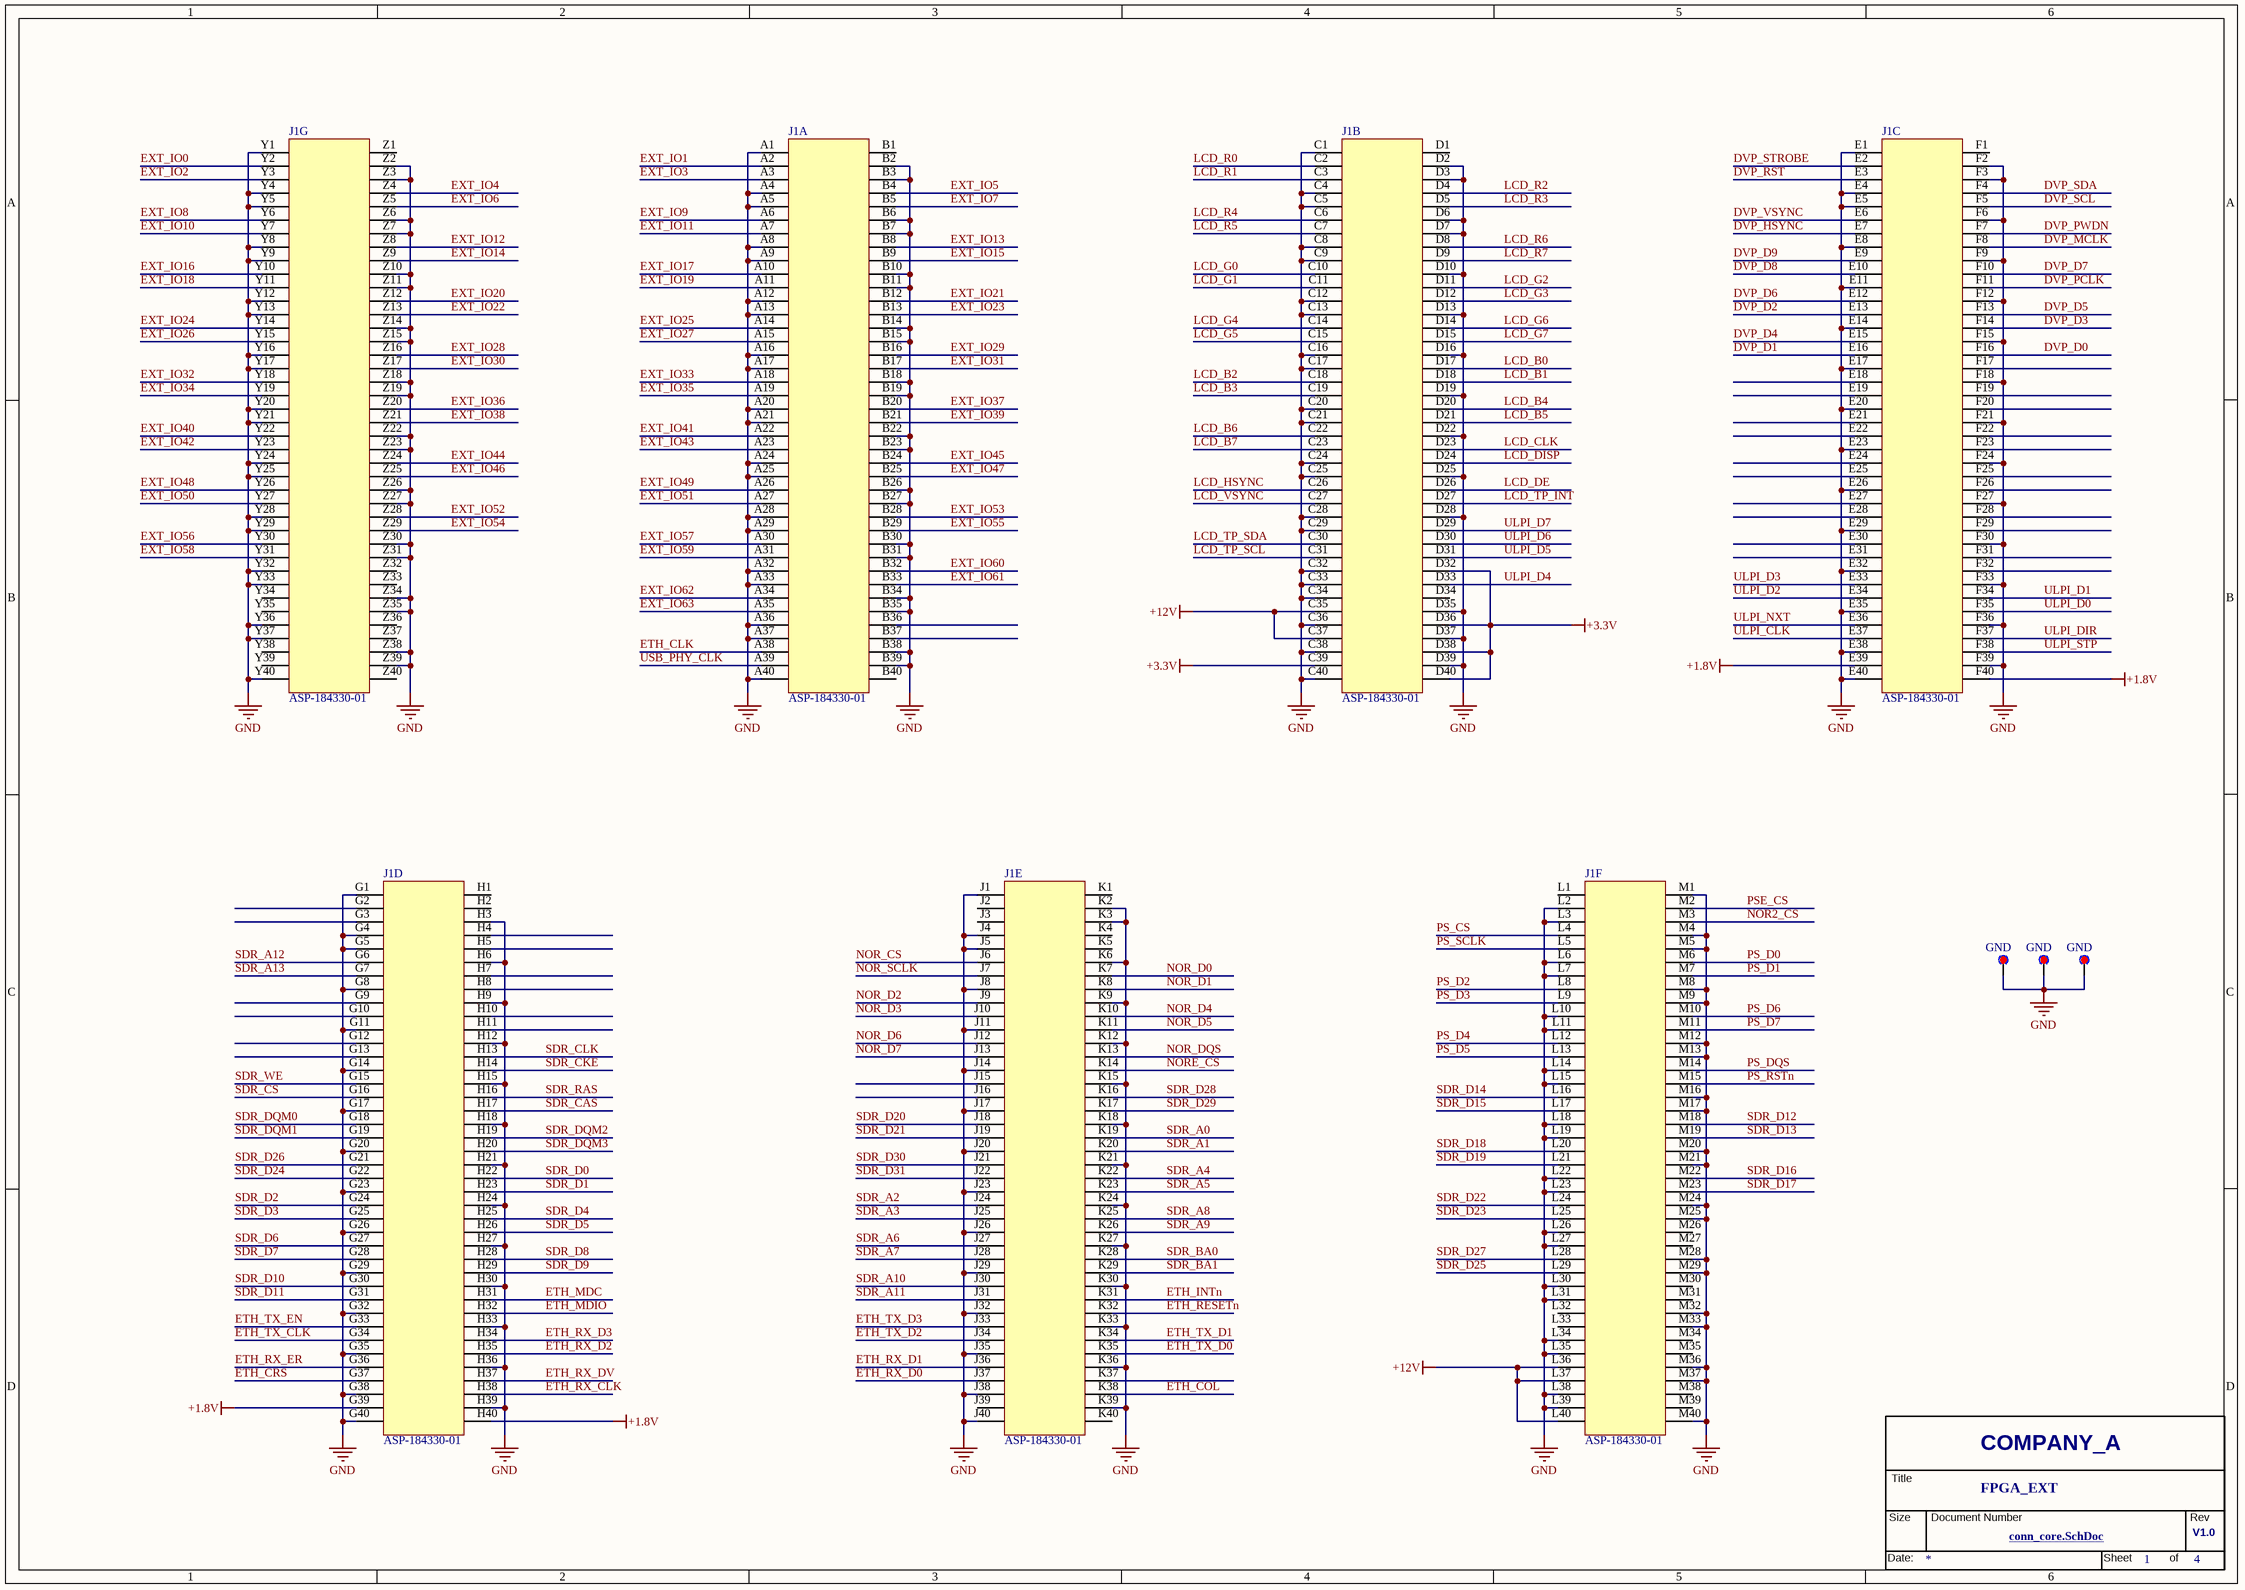
[diagram p0: MISC105414-3.SchDoc]
# Altium project MISC105414-4.PrjPcb (part 1 of 3)
4 sheets, 256 parts. Net scope: global (net labels, ports and power ports of the same name join across sheets).
Board file: MISC105414.PcbDoc
Sheets:
  MISC105414-3.SchDoc
  MISC105414-2.SchDoc
  MISC105414-7.SchDoc
  MISC105414-8.SchDoc

## Sheet MISC105414-3.SchDoc
size 420 x 297 mm; DocumentNumber: MISC105414; SheetNumber: 1; SheetTotal: 4

### Parts
(Parts that share a designator on the sheet are numbered #1, #2 ... from top to bottom, then left to right.)
*?#1  Page Count: 4  Page Number: 1  OrgName: COMPANY_A  Title: FPGA_EXT  RevCode: V1.0  Doc: conn_core.SchDoc  (hidden comment: TitleBlock_YHSCH)  (graphical)
J1  ASP-184330-01  [ASP-184330-01_Bottom]  (parts A,B,C,D,E,F,G of 7)
TP1  GND  [FZ_TP-Via]
TP2  GND  [FZ_TP-Via]
TP3  GND  [FZ_TP-Via]

### Nets
+1.8V: J1.E39(P) J1.F40(P) J1.G39(P) J1.H40(P)
+3.3V: J1.C39(P) J1.D32(P) J1.D36(P) J1.D38(P) J1.D40(P)
+12V: J1.C35(P) J1.C37(P) J1.L36(P) J1.L37(P) J1.L40(P)
GND: J1.A1(P) J1.A4(P) J1.A5(P) J1.A8(P) J1.A9(P) J1.A12(P) J1.A13(P) J1.A16(P) J1.A17(P) J1.A20(P) J1.A21(P) J1.A24(P) J1.A25(P) J1.A28(P) J1.A29(P) J1.A32(P) J1.A33(P) J1.A36(P) J1.A37(P) J1.A40(P) J1.B2(P) J1.B3(P) J1.B6(P) J1.B7(P) J1.B10(P) J1.B11(P) J1.B14(P) J1.B15(P) J1.B18(P) J1.B19(P) J1.B22(P) J1.B23(P) J1.B26(P) J1.B27(P) J1.B30(P) J1.B31(P) J1.B34(P) J1.B35(P) J1.B38(P) J1.B39(P) J1.C1(P) J1.C4(P) J1.C5(P) J1.C8(P) J1.C9(P) J1.C12(P) J1.C13(P) J1.C16(P) J1.C17(P) J1.C20(P) J1.C21(P) J1.C24(P) J1.C25(P) J1.C28(P) J1.C29(P) J1.C32(P) J1.C33(P) J1.C34(P) J1.C36(P) J1.C38(P) J1.C40(P) J1.D2(P) J1.D3(P) J1.D6(P) J1.D7(P) J1.D10(P) J1.D13(P) J1.D16(P) J1.D19(P) J1.D22(P) J1.D25(P) J1.D28(P) J1.D35(P) J1.D37(P) J1.D39(P) J1.E1(P) J1.E4(P) J1.E5(P) J1.E8(P) J1.E11(P) J1.E14(P) J1.E17(P) J1.E20(P) J1.E23(P) J1.E26(P) J1.E29(P) J1.E32(P) J1.E35(P) J1.E38(P) J1.E40(P) J1.F2(P) J1.F3(P) J1.F6(P) J1.F9(P) J1.F12(P) J1.F15(P) J1.F18(P) J1.F21(P) J1.F24(P) J1.F27(P) J1.F30(P) J1.F33(P) J1.F36(P) J1.F39(P) J1.G1(P) J1.G4(P) J1.G5(P) J1.G8(P) J1.G11(P) J1.G14(P) J1.G17(P) J1.G20(P) J1.G23(P) J1.G26(P) J1.G29(P) J1.G32(P) J1.G35(P) J1.G38(P) J1.G40(P) J1.H3(P) J1.H6(P) J1.H9(P) J1.H12(P) J1.H15(P) J1.H18(P) J1.H21(P) J1.H24(P) J1.H27(P) J1.H30(P) J1.H33(P) J1.H36(P) J1.H39(P) J1.J1(P) J1.J4(P) J1.J5(P) J1.J8(P) J1.J11(P) J1.J14(P) J1.J17(P) J1.J20(P) J1.J23(P) J1.J26(P) J1.J29(P) J1.J32(P) J1.J35(P) J1.J38(P) J1.J40(P) J1.K2(P) J1.K3(P) J1.K6(P) J1.K9(P) J1.K12(P) J1.K15(P) J1.K18(P) J1.K21(P) J1.K24(P) J1.K27(P) J1.K30(P) J1.K33(P) J1.K36(P) J1.K39(P) J1.L2(P) J1.L3(P) J1.L6(P) J1.L7(P) J1.L10(P) J1.L11(P) J1.L14(P) J1.L15(P) J1.L18(P) J1.L19(P) J1.L22(P) J1.L23(P) J1.L26(P) J1.L27(P) J1.L30(P) J1.L31(P) J1.L34(P) J1.L35(P) J1.L38(P) J1.L39(P) J1.M1(P) J1.M4(P) J1.M5(P) J1.M8(P) J1.M9(P) J1.M12(P) J1.M13(P) J1.M16(P) J1.M17(P) J1.M20(P) J1.M21(P) J1.M24(P) J1.M25(P) J1.M28(P) J1.M29(P) J1.M32(P) J1.M33(P) J1.M36(P) J1.M37(P) J1.M40(P) J1.Y1(P) J1.Y4(P) J1.Y5(P) J1.Y8(P) J1.Y9(P) J1.Y12(P) J1.Y13(P) J1.Y16(P) J1.Y17(P) J1.Y20(P) J1.Y21(P) J1.Y24(P) J1.Y25(P) J1.Y28(P) J1.Y29(P) J1.Y32(P) J1.Y33(P) J1.Y36(P) J1.Y37(P) J1.Y40(P) J1.Z2(P) J1.Z3(P) J1.Z6(P) J1.Z7(P) J1.Z10(P) J1.Z11(P) J1.Z14(P) J1.Z15(P) J1.Z18(P) J1.Z19(P) J1.Z22(P) J1.Z23(P) J1.Z26(P) J1.Z27(P) J1.Z30(P) J1.Z31(P) J1.Z34(P) J1.Z35(P) J1.Z38(P) J1.Z39(P) TP1.1 TP2.1 TP3.1
DVP_D0: J1.F16(P)
DVP_D1: J1.E16(P)
DVP_D2: J1.E13(P)
DVP_D3: J1.F14(P)
DVP_D4: J1.E15(P)
DVP_D5: J1.F13(P)
DVP_D6: J1.E12(P)
DVP_D7: J1.F10(P)
DVP_D8: J1.E10(P)
DVP_D9: J1.E9(P)
DVP_HSYNC: J1.E7(P)
DVP_MCLK: J1.F8(P)
DVP_PCLK: J1.F11(P)
DVP_PWDN: J1.F7(P)
DVP_RST: J1.E3(P)
DVP_SCL: J1.F5(P)
DVP_SDA: J1.F4(P)
DVP_STROBE: J1.E2(P)
DVP_VSYNC: J1.E6(P)
ETH_CLK: J1.A38(P)
ETH_COL: J1.K38(P)
ETH_CRS: J1.G37(P)
ETH_INTn: J1.K31(P)
ETH_MDC: J1.H31(P)
ETH_MDIO: J1.H32(P)
ETH_RESETn: J1.K32(P)
ETH_RX_CLK: J1.H38(P)
ETH_RX_D0: J1.J37(P)
ETH_RX_D1: J1.J36(P)
ETH_RX_D2: J1.H35(P)
ETH_RX_D3: J1.H34(P)
ETH_RX_DV: J1.H37(P)
ETH_RX_ER: J1.G36(P)
ETH_TX_CLK: J1.G34(P)
ETH_TX_D0: J1.K35(P)
ETH_TX_D1: J1.K34(P)
ETH_TX_D2: J1.J34(P)
ETH_TX_D3: J1.J33(P)
ETH_TX_EN: J1.G33(P)
EXT_IO0: J1.Y2(P)
EXT_IO1: J1.A2(P)
EXT_IO2: J1.Y3(P)
EXT_IO3: J1.A3(P)
EXT_IO4: J1.Z4(P)
EXT_IO5: J1.B4(P)
EXT_IO6: J1.Z5(P)
EXT_IO7: J1.B5(P)
EXT_IO8: J1.Y6(P)
EXT_IO9: J1.A6(P)
EXT_IO10: J1.Y7(P)
EXT_IO11: J1.A7(P)
EXT_IO12: J1.Z8(P)
EXT_IO13: J1.B8(P)
EXT_IO14: J1.Z9(P)
EXT_IO15: J1.B9(P)
EXT_IO16: J1.Y10(P)
EXT_IO17: J1.A10(P)
EXT_IO18: J1.Y11(P)
EXT_IO19: J1.A11(P)
EXT_IO20: J1.Z12(P)
EXT_IO21: J1.B12(P)
EXT_IO22: J1.Z13(P)
EXT_IO23: J1.B13(P)
EXT_IO24: J1.Y14(P)
EXT_IO25: J1.A14(P)
EXT_IO26: J1.Y15(P)
EXT_IO27: J1.A15(P)
EXT_IO28: J1.Z16(P)
EXT_IO29: J1.B16(P)
EXT_IO30: J1.Z17(P)
EXT_IO31: J1.B17(P)
EXT_IO32: J1.Y18(P)
EXT_IO33: J1.A18(P)
EXT_IO34: J1.Y19(P)
EXT_IO35: J1.A19(P)
EXT_IO36: J1.Z20(P)
EXT_IO37: J1.B20(P)
EXT_IO38: J1.Z21(P)
EXT_IO39: J1.B21(P)
EXT_IO40: J1.Y22(P)
EXT_IO41: J1.A22(P)
EXT_IO42: J1.Y23(P)
EXT_IO43: J1.A23(P)
EXT_IO44: J1.Z24(P)
EXT_IO45: J1.B24(P)
EXT_IO46: J1.Z25(P)
EXT_IO47: J1.B25(P)
EXT_IO48: J1.Y26(P)
EXT_IO49: J1.A26(P)
EXT_IO50: J1.Y27(P)
EXT_IO51: J1.A27(P)
EXT_IO52: J1.Z28(P)
EXT_IO53: J1.B28(P)
EXT_IO54: J1.Z29(P)
EXT_IO55: J1.B29(P)
EXT_IO56: J1.Y30(P)
EXT_IO57: J1.A30(P)
EXT_IO58: J1.Y31(P)
EXT_IO59: J1.A31(P)
EXT_IO60: J1.B32(P)
EXT_IO61: J1.B33(P)
EXT_IO62: J1.A34(P)
EXT_IO63: J1.A35(P)
LCD_B0: J1.D17(P)
LCD_B1: J1.D18(P)
LCD_B2: J1.C18(P)
LCD_B3: J1.C19(P)
LCD_B4: J1.D20(P)
LCD_B5: J1.D21(P)
LCD_B6: J1.C22(P)
LCD_B7: J1.C23(P)
LCD_CLK: J1.D23(P)
LCD_DE: J1.D26(P)
LCD_DISP: J1.D24(P)
LCD_G0: J1.C10(P)
LCD_G1: J1.C11(P)
LCD_G2: J1.D11(P)
LCD_G3: J1.D12(P)
LCD_G4: J1.C14(P)
LCD_G5: J1.C15(P)
LCD_G6: J1.D14(P)
LCD_G7: J1.D15(P)
LCD_HSYNC: J1.C26(P)
LCD_R0: J1.C2(P)
LCD_R1: J1.C3(P)
LCD_R2: J1.D4(P)
LCD_R3: J1.D5(P)
LCD_R4: J1.C6(P)
LCD_R5: J1.C7(P)
LCD_R6: J1.D8(P)
LCD_R7: J1.D9(P)
LCD_TP_INT: J1.D27(P)
LCD_TP_SCL: J1.C31(P)
LCD_TP_SDA: J1.C30(P)
LCD_VSYNC: J1.C27(P)
NOR2_CS: J1.M3(P)
NOR_CS: J1.J6(P)
NOR_D0: J1.K7(P)
NOR_D1: J1.K8(P)
NOR_D2: J1.J9(P)
NOR_D3: J1.J10(P)
NOR_D4: J1.K10(P)
NOR_D5: J1.K11(P)
NOR_D6: J1.J12(P)
NOR_D7: J1.J13(P)
NOR_DQS: J1.K13(P)
NOR_SCLK: J1.J7(P)
NORE_CS: J1.K14(P)
PS_CS: J1.L4(P)
PS_D0: J1.M6(P)
PS_D1: J1.M7(P)
PS_D2: J1.L8(P)
PS_D3: J1.L9(P)
PS_D4: J1.L12(P)
PS_D5: J1.L13(P)
PS_D6: J1.M10(P)
PS_D7: J1.M11(P)
PS_DQS: J1.M14(P)
PS_RSTn: J1.M15(P)
PS_SCLK: J1.L5(P)
PSE_CS: J1.M2(P)
SDR_A0: J1.K19(P)
SDR_A1: J1.K20(P)
SDR_A2: J1.J24(P)
SDR_A3: J1.J25(P)
SDR_A4: J1.K22(P)
SDR_A5: J1.K23(P)
SDR_A6: J1.J27(P)
SDR_A7: J1.J28(P)
SDR_A8: J1.K25(P)
SDR_A9: J1.K26(P)
SDR_A10: J1.J30(P)
SDR_A11: J1.J31(P)
SDR_A12: J1.G6(P)
SDR_A13: J1.G7(P)
SDR_BA0: J1.K28(P)
SDR_BA1: J1.K29(P)
SDR_CAS: J1.H17(P)
SDR_CKE: J1.H14(P)
SDR_CLK: J1.H13(P)
SDR_CS: J1.G16(P)
SDR_D0: J1.H22(P)
SDR_D1: J1.H23(P)
SDR_D2: J1.G24(P)
SDR_D3: J1.G25(P)
SDR_D4: J1.H25(P)
SDR_D5: J1.H26(P)
SDR_D6: J1.G27(P)
SDR_D7: J1.G28(P)
SDR_D8: J1.H28(P)
SDR_D9: J1.H29(P)
SDR_D10: J1.G30(P)
SDR_D11: J1.G31(P)
SDR_D12: J1.M18(P)
SDR_D13: J1.M19(P)
SDR_D14: J1.L16(P)
SDR_D15: J1.L17(P)
SDR_D16: J1.M22(P)
SDR_D17: J1.M23(P)
SDR_D18: J1.L20(P)
SDR_D19: J1.L21(P)
SDR_D20: J1.J18(P)
SDR_D21: J1.J19(P)
SDR_D22: J1.L24(P)
SDR_D23: J1.L25(P)
SDR_D24: J1.G22(P)
SDR_D25: J1.L29(P)
SDR_D26: J1.G21(P)
SDR_D27: J1.L28(P)
SDR_D28: J1.K16(P)
SDR_D29: J1.K17(P)
SDR_D30: J1.J21(P)
SDR_D31: J1.J22(P)
SDR_DQM0: J1.G18(P)
SDR_DQM1: J1.G19(P)
SDR_DQM2: J1.H19(P)
SDR_DQM3: J1.H20(P)
SDR_RAS: J1.H16(P)
SDR_WE: J1.G15(P)
ULPI_CLK: J1.E37(P)
ULPI_D0: J1.F35(P)
ULPI_D1: J1.F34(P)
ULPI_D2: J1.E34(P)
ULPI_D3: J1.E33(P)
ULPI_D4: J1.D33(P)
ULPI_D5: J1.D31(P)
ULPI_D6: J1.D30(P)
ULPI_D7: J1.D29(P)
ULPI_DIR: J1.F37(P)
ULPI_NXT: J1.E36(P)
ULPI_STP: J1.F38(P)
USB_PHY_CLK: J1.A39(P)

Not connected (* = marked no-connect by the designer): J1 B1(P) B36(P) B37(P) B40(P) D1(P) D34(P) E18(P) E19(P) E21(P) E22(P) E24(P) E25(P) E27(P) E28(P) E30(P) E31(P) F1(P) F17(P) F19(P) F20(P) F22(P) F23(P) F25(P) F26(P) F28(P) F29(P) F31(P) F32(P) G2(P) G3(P) G9(P) G10(P) G12(P) G13(P) H1(P) H2(P) H4(P) H5(P) H7(P) H8(P) H10(P) H11(P) J2(P) J3(P) J15(P) J16(P) J39(P) K1(P) K4(P) K5(P) K37(P) K40(P) L1(P) L32(P) L33(P) M26(P) M27(P) M30(P) M31(P) M34(P) M35(P) M38(P) M39(P) Y34(P) Y35(P) Y38(P) Y39(P) Z1(P) Z32(P) Z33(P) Z36(P) Z37(P) Z40(P)

### Library data of the parts
J1 = ASP-184329-01
TP1-TP3 = TP_SMD
*?#1 = TitleBlock_YHSCH: Page Modify Date: *; Cage Code: 1

## Sheet MISC105414-2.SchDoc
size 420 x 297 mm; DocumentNumber: MISC105414; SheetNumber: 3; SheetTotal: 4
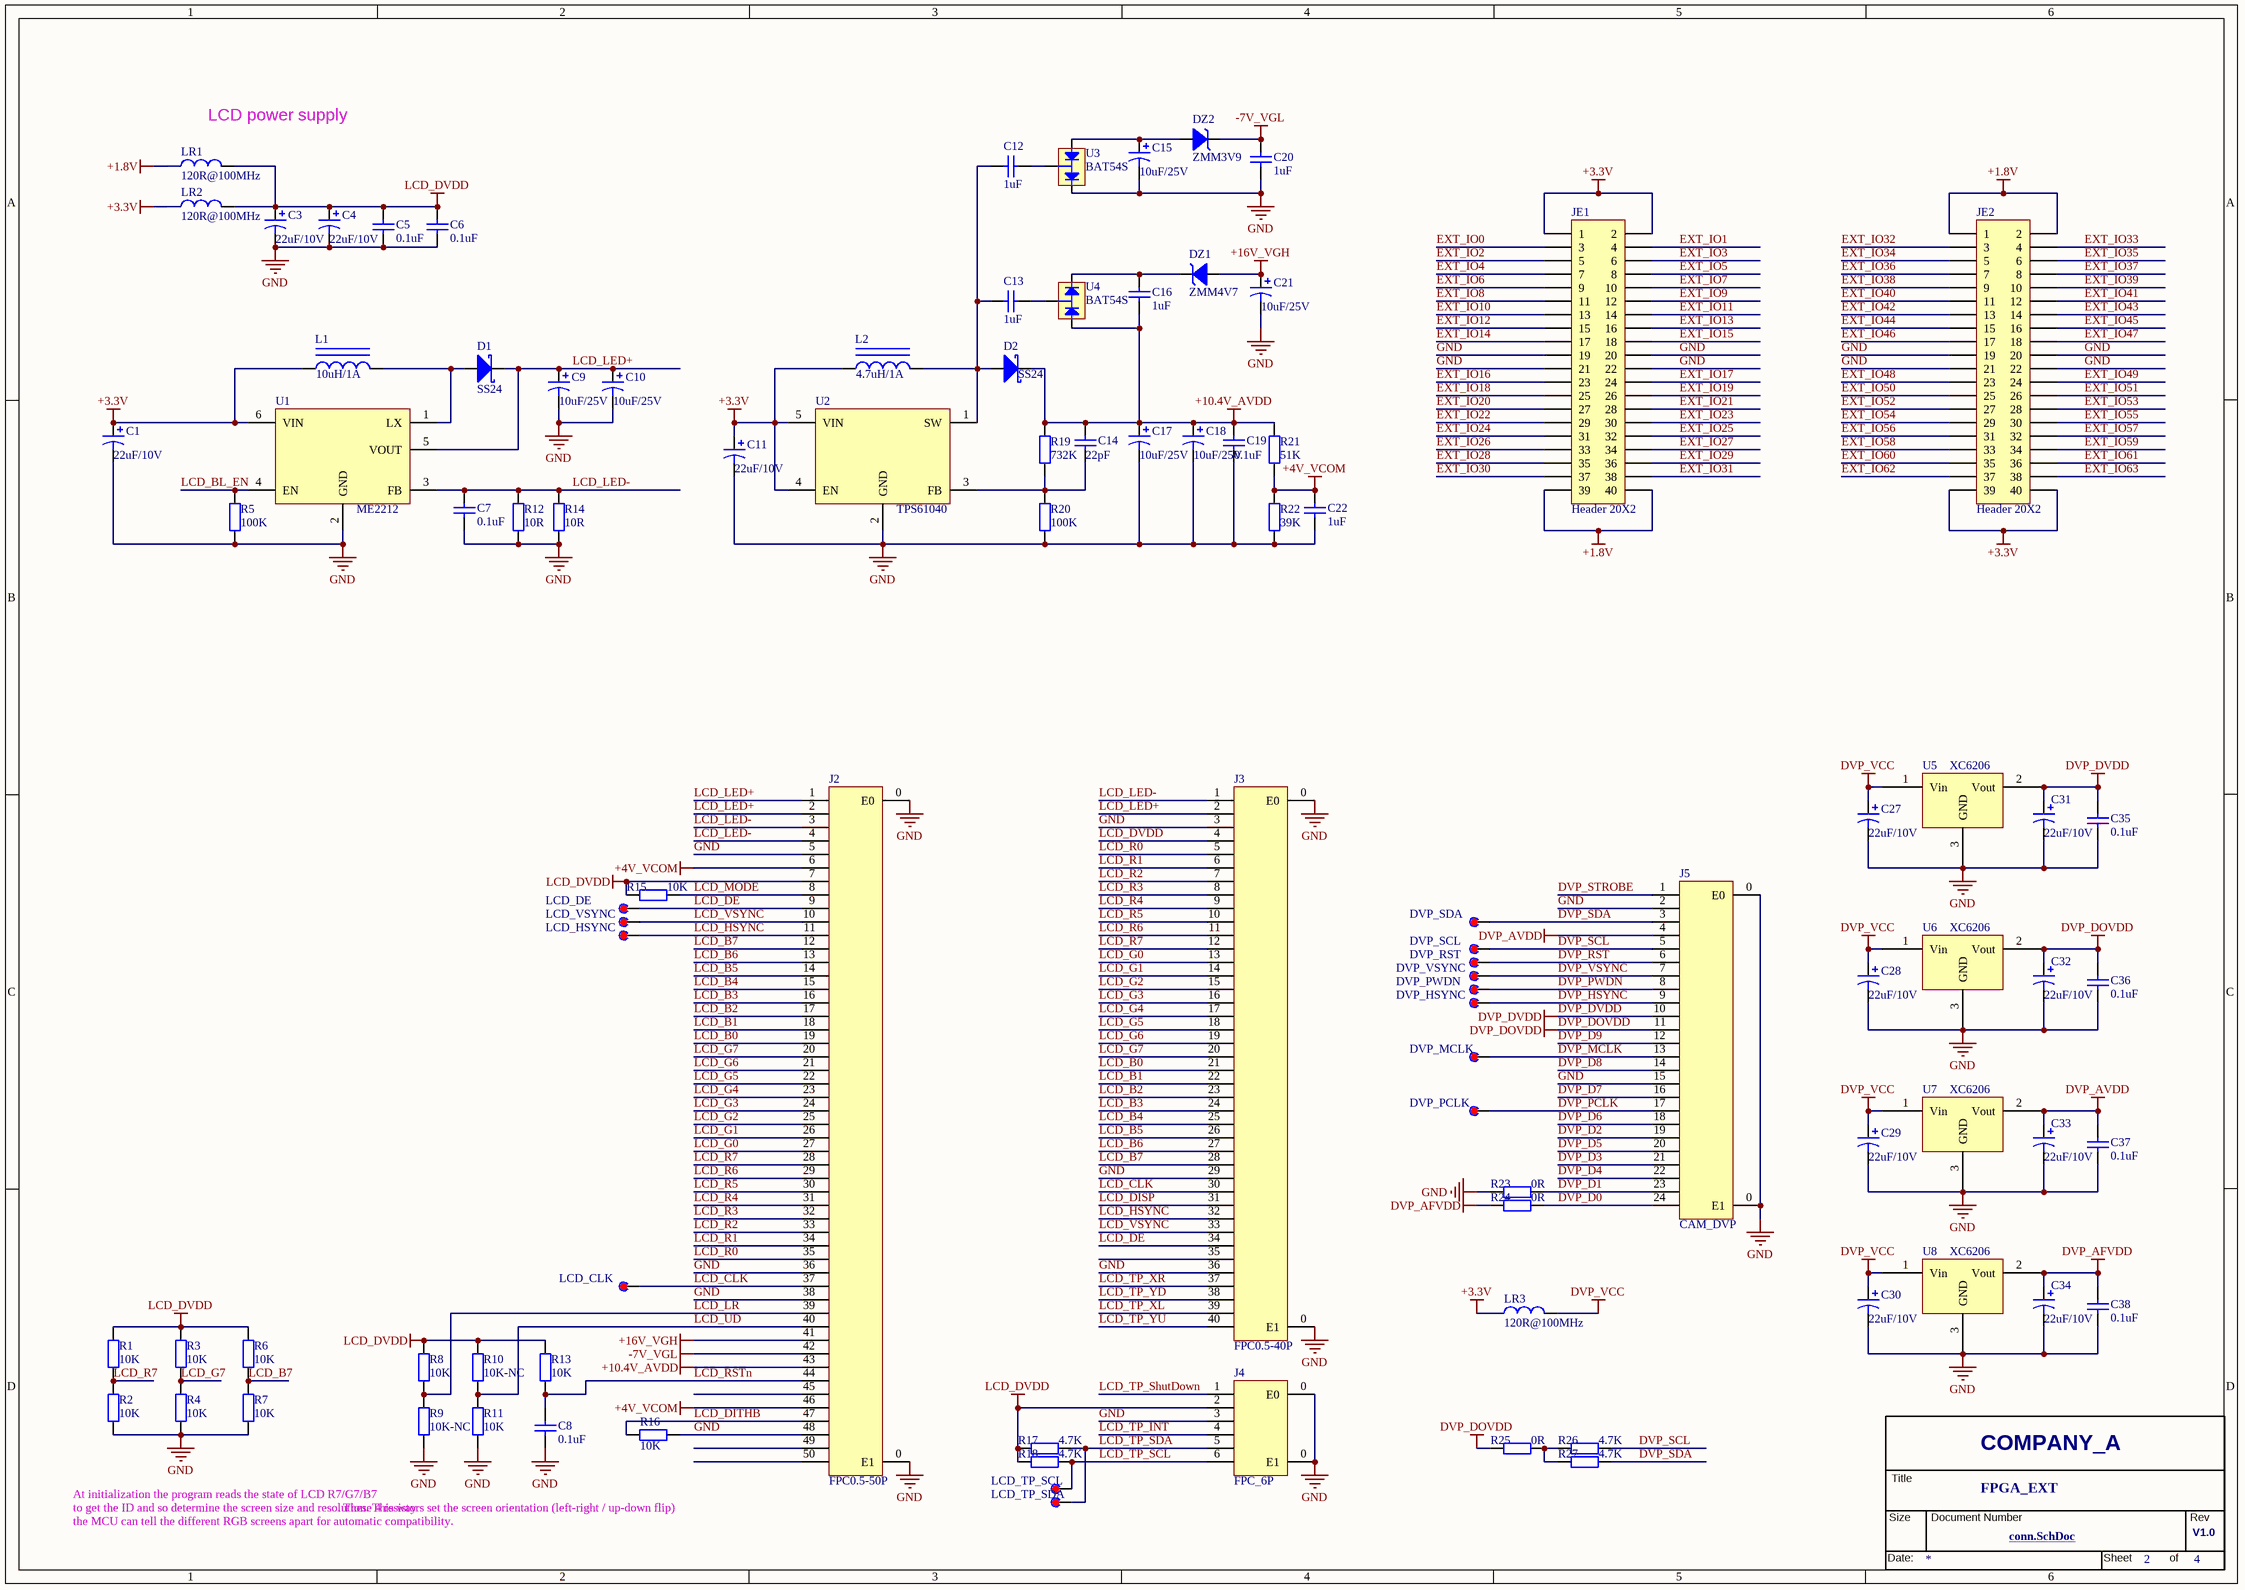
[diagram p1: MISC105414-2.SchDoc]

### Parts
(Parts that share a designator on the sheet are numbered #1, #2 ... from top to bottom, then left to right.)
*?#2  Page Count: 4  Page Number: 2  OrgName: COMPANY_A  Title: FPGA_EXT  RevCode: V1.0  Doc: conn.SchDoc  (hidden comment: TitleBlock_YHSCH)  (graphical)
C1  22uF/10V  [0603C_N]
C3  22uF/10V  [0603C_N]
C4  22uF/10V  [0603C_N]
C5  0.1uF  [0603C_N]
C6  0.1uF  [0603C_N]
C7  0.1uF  [0603C_N]
C8  0.1uF  [0603C_N]
C9  10uF/25V  [0603C_N]
C10  10uF/25V  [0603C_N]
C11  22uF/10V  [0603C_N]
C12  1uF  [0603C_N]
C13  1uF  [0603C_N]
C14  22pF  [0603C_N]
C15  10uF/25V  [0603C_N]
C16  1uF  [0603C_N]
C17  10uF/25V  [0603C_N]
C18  10uF/25V  [0603C_N]
C19  0.1uF  [0603C_N]
C20  1uF  [0603C_N]
C21  10uF/25V  [0603C_N]
C22  1uF  [0603C_N]
C27  22uF/10V  [0603C_N]
C28  22uF/10V  [0603C_N]
C29  22uF/10V  [0603C_N]
C30  22uF/10V  [0603C_N]
C31  22uF/10V  [0603C_N]
C32  22uF/10V  [0603C_N]
C33  22uF/10V  [0603C_N]
C34  22uF/10V  [0603C_N]
C35  0.1uF  [0603C_N]
C36  0.1uF  [0603C_N]
C37  0.1uF  [0603C_N]
C38  0.1uF  [0603C_N]
D1  SS24  [DO-214AC]
D2  SS24  [DO-214AC]
DZ1  ZMM4V7  [LL-34]
DZ2  ZMM3V9  [LL-34]
J2  FPC0.5-50P  [FPC0.5-50P]
J3  FPC0.5-40P  [FPC0.5-40P]
J4  FPC_6P  [FPC0.5-6P]
J5  CAM_DVP  [FPC0.5-24P]
JE1  Header 20X2  [HDR2X20]
JE2  Header 20X2  [HDR2X20]
L1  10uH/1A  [LD-5.5mm]
L2  4.7uH/1A  [LD-5.5mm]
LR1  120R@100MHz  [0603R_N]
LR2  120R@100MHz  [0603R_N]
LR3  120R@100MHz  [0603R_N]
R1  10K  [0603R_N]
R2  10K  [0603R_N]
R3  10K  [0603R_N]
R4  10K  [0603R_N]
R5  100K  [0603R_N]
R6  10K  [0603R_N]
R7  10K  [0603R_N]
R8  10K  [0603R_N]
R9  10K-NC  [0603R_N]
R10  10K-NC  [0603R_N]
R11  10K  [0603R_N]
R12  10R  [0603R_N]
R13  10K  [0603R_N]
R14  10R  [0603R_N]
R15  10K  [0603R_N]
R16  10K  [0603R_N]
R17  4.7K  [0603R_N]
R18  4.7K  [0603R_N]
R19  732K  [0603R_N]
R20  100K  [0603R_N]
R21  51K  [0603R_N]
R22  39K  [0603R_N]
R23  0R  [0603R_N]
R24  0R  [0603R_N]
R25  0R  [0603R_N]
R26  4.7K  [0603R_N]
R27  4.7K  [0603R_N]
TP4  LCD_DE  [FZ_TP-SMD-Mini]
TP5  LCD_VSYNC  [FZ_TP-SMD-Mini]
TP6  LCD_HSYNC  [FZ_TP-SMD-Mini]
TP7  LCD_CLK  [FZ_TP-SMD-Mini]
TP8  LCD_TP_SCL  [FZ_TP-SMD-Mini]
TP9  LCD_TP_SDA  [FZ_TP-SMD-Mini]
TP10  DVP_VSYNC  [FZ_TP-SMD-Mini]
TP11  DVP_PWDN  [FZ_TP-SMD-Mini]
TP12  DVP_HSYNC  [FZ_TP-SMD-Mini]
TP13  DVP_SDA  [FZ_TP-SMD-Mini]
TP14  DVP_SCL  [FZ_TP-SMD-Mini]
TP15  DVP_RST  [FZ_TP-SMD-Mini]
TP16  DVP_MCLK  [FZ_TP-SMD-Mini]
TP17  DVP_PCLK  [FZ_TP-SMD-Mini]
U1  ME2212  [SOT-23-6]
U2  TPS61040  [SOT-23-5]
U3  BAT54S  [SOT-23]
U4  BAT54S  [SOT-23]
U5  XC6206  [SOT-23]
U6  XC6206  [SOT-23]
U7  XC6206  [SOT-23]
U8  XC6206  [SOT-23]

### Nets
+1.8V: JE1.39 JE1.40 JE2.1 JE2.2 LR1.2
+3.3V: C1.1 C11.1 JE1.1 JE1.2 JE2.39 JE2.40 L1.1 L2.1 LR2.2 LR3.2 U1.6(VIN) U2.4(EN) U2.5(VIN)
+4V_VCOM: C22.1 J2.6 J2.46 R21.1 R22.2
+10.4V_AVDD: C14.2 C16.2 C17.1 C18.1 C19.2 D2.2(K) J2.43 R19.2 R21.2 U4.1
+16V_VGH: C21.1 DZ1.1(K) J2.41
-7V_VGL: C20.1 DZ2.2(A) J2.42
DVP_AFVDD: C34.1 C38.2 R24.1 U8.2(Vout)
DVP_AVDD: C33.1 C37.2 J5.4 U7.2(Vout)
DVP_DOVDD: C32.1 C36.2 J5.11 R25.1 U6.2(Vout)
DVP_DVDD: C31.1 C35.2 J5.10 U5.2(Vout)
DVP_VCC: C27.1 C28.1 C29.1 C30.1 LR3.1 U5.1(Vin) U6.1(Vin) U7.1(Vin) U8.1(Vin)
GND: C1.2 C3.2 C4.2 C5.1 C6.1 C7.1 C8.1 C9.2 C10.2 C11.2 C15.2 C17.2 C18.2 C19.1 C20.2 C21.2 C22.2 C27.2 C28.2 C29.2 C30.2 C31.2 C32.2 C33.2 C34.2 C35.1 C36.1 C37.1 C38.1 J2.0(E0) J2.5 J2.36 J2.38 J2.48 J3.0(E0) J3.3 J3.29 J3.36 J4.0(E0) J4.3 J5.0(E0) J5.2 J5.15 JE1.19 JE1.20 JE1.21 JE1.22 JE2.19 JE2.20 JE2.21 JE2.22 R2.1 R4.1 R5.1 R7.1 R9.1 R11.1 R12.1 R14.1 R16.1 R20.1 R22.1 R23.1 U1.2(GND) U2.2(GND) U3.2 U5.3(GND) U6.3(GND) U7.3(GND) U8.3(GND)
LCD_DVDD: C3.1 C4.1 C5.2 C6.2 J2.7 J3.4 J4.2 LR1.1 LR2.1 R1.2 R3.2 R6.2 R8.2 R10.2 R13.2 R15.2 R17.2 R18.2
DVP_D0: J5.24 R24.2
DVP_D1: J5.23 R23.2
DVP_D2: J5.19
DVP_D3: J5.21
DVP_D4: J5.22
DVP_D5: J5.20
DVP_D6: J5.18
DVP_D7: J5.16
DVP_D8: J5.14
DVP_D9: J5.12
DVP_HSYNC: J5.9 TP12.1
DVP_MCLK: J5.13 TP16.1
DVP_PCLK: J5.17 TP17.1
DVP_PWDN: J5.8 TP11.1
DVP_RST: J5.6 TP15.1
DVP_SCL: J5.5 R26.1 TP14.1
DVP_SDA: J5.3 R27.1 TP13.1
DVP_STROBE: J5.1
DVP_VSYNC: J5.7 TP10.1
EXT_IO0: JE1.3
EXT_IO1: JE1.4
EXT_IO2: JE1.5
EXT_IO3: JE1.6
EXT_IO4: JE1.7
EXT_IO5: JE1.8
EXT_IO6: JE1.9
EXT_IO7: JE1.10
EXT_IO8: JE1.11
EXT_IO9: JE1.12
EXT_IO10: JE1.13
EXT_IO11: JE1.14
EXT_IO12: JE1.15
EXT_IO13: JE1.16
EXT_IO14: JE1.17
EXT_IO15: JE1.18
EXT_IO16: JE1.23
EXT_IO17: JE1.24
EXT_IO18: JE1.25
EXT_IO19: JE1.26
EXT_IO20: JE1.27
EXT_IO21: JE1.28
EXT_IO22: JE1.29
EXT_IO23: JE1.30
EXT_IO24: JE1.31
EXT_IO25: JE1.32
EXT_IO26: JE1.33
EXT_IO27: JE1.34
EXT_IO28: JE1.35
EXT_IO29: JE1.36
EXT_IO30: JE1.37
EXT_IO31: JE1.38
EXT_IO32: JE2.3
EXT_IO33: JE2.4
EXT_IO34: JE2.5
EXT_IO35: JE2.6
EXT_IO36: JE2.7
EXT_IO37: JE2.8
EXT_IO38: JE2.9
EXT_IO39: JE2.10
EXT_IO40: JE2.11
EXT_IO41: JE2.12
EXT_IO42: JE2.13
EXT_IO43: JE2.14
EXT_IO44: JE2.15
EXT_IO45: JE2.16
EXT_IO46: JE2.17
EXT_IO47: JE2.18
EXT_IO48: JE2.23
EXT_IO49: JE2.24
EXT_IO50: JE2.25
EXT_IO51: JE2.26
EXT_IO52: JE2.27
EXT_IO53: JE2.28
EXT_IO54: JE2.29
EXT_IO55: JE2.30
EXT_IO56: JE2.31
EXT_IO57: JE2.32
EXT_IO58: JE2.33
EXT_IO59: JE2.34
EXT_IO60: JE2.35
EXT_IO61: JE2.36
EXT_IO62: JE2.37
EXT_IO63: JE2.38
LCD_B0: J2.19 J3.21
LCD_B1: J2.18 J3.22
LCD_B2: J2.17 J3.23
LCD_B3: J2.16 J3.24
LCD_B4: J2.15 J3.25
LCD_B5: J2.14 J3.26
LCD_B6: J2.13 J3.27
LCD_B7: J2.12 J3.28 R6.1 R7.2
LCD_BL_EN: R5.2 U1.4(EN)
LCD_CLK: J2.37 J3.30 TP7.1
LCD_DE: J2.9 J3.34 TP4.1
LCD_DISP: J3.31
LCD_DITHB: J2.47 R16.2
LCD_G0: J2.27 J3.13
LCD_G1: J2.26 J3.14
LCD_G2: J2.25 J3.15
LCD_G3: J2.24 J3.16
LCD_G4: J2.23 J3.17
LCD_G5: J2.22 J3.18
LCD_G6: J2.21 J3.19
LCD_G7: J2.20 J3.20 R3.1 R4.2
LCD_HSYNC: J2.11 J3.32 TP6.1
LCD_LED+: C9.1 C10.1 D1.2(K) J2.1 J2.2 J3.2 U1.5(VOUT)
LCD_LED-: C7.2 J2.3 J2.4 J3.1 R12.2 R14.2 U1.3(FB)
LCD_LR: J2.39 R8.1 R9.2
LCD_MODE: J2.8 R15.1
LCD_R0: J2.35 J3.5
LCD_R1: J2.34 J3.6
LCD_R2: J2.33 J3.7
LCD_R3: J2.32 J3.8
LCD_R4: J2.31 J3.9
LCD_R5: J2.30 J3.10
LCD_R6: J2.29 J3.11
LCD_R7: J2.28 J3.12 R1.1 R2.2
LCD_RSTn: C8.2 J2.44 R13.1
LCD_TP_INT: J4.4
LCD_TP_SCL: J4.6 R18.1 TP8.1
LCD_TP_SDA: J4.5 R17.1 TP9.1
LCD_TP_ShutDown: J4.1
LCD_TP_XL: J3.39
LCD_TP_XR: J3.37
LCD_TP_YD: J3.38
LCD_TP_YU: J3.40
LCD_UD: J2.40 R10.1 R11.2
LCD_VSYNC: J2.10 J3.33 TP5.1
NetC12_1: C12.1 U3.3
NetC12_2: C12.2 C13.2 D2.1(A) L2.2 U2.1(SW)
NetC13_1: C13.1 U4.3
NetC14_1: C14.1 R19.1 R20.2 U2.3(FB)
NetC15_1: C15.1 DZ2.1(K) U3.1
NetC16_1: C16.1 DZ1.2(A) U4.2
NetD1_1: D1.1(A) L1.2 U1.1(LX)
NetR25_2: R25.2 R26.2 R27.2

Not connected (* = marked no-connect by the designer): J2 45 49 50; J3 35

### Notes on the sheet
- (near LR1) LCD power supply
- At initialization the program reads the state of LCD R7/G7/B7
- to get the ID and so determine the screen size and resolution. This way
- the MCU can tell the different RGB screens apart for automatic compatibility.
- These 4 resistors set the screen orientation (left-right / up-down flip)

### Library data of the parts
*?#2 = TitleBlock_YHSCH: Cage Code: 1; Page Modify Date: *
C1 C3 C4 C9-C11 C15 C17 C18 C21 C27-C34 = Cap Pol1: Polarized Capacitor (Radial); Value: 1uF; Published: 8-Jun-2000; LatestRevisionDate: 17-Jul-2002; LatestRevisionNote: Re-released for DXP Platform.; PackageReference: RB7.6-15; Publisher: Altium Limited
C5-C8 C12-C14 C16 C19 C20 C22 C35-C38 = Cap: Capacitor; Value: 100nF; Published: 8-Jun-2000; LatestRevisionDate: 17-Jul-2002; LatestRevisionNote: Re-released for DXP Platform.; PackageReference: RAD-0.3; Publisher: Altium Limited
D1 D2 = Diode BAS70: Silicon AF Schottky Diode for High-Speed Switching; Note: Pin 2 is not connected and not drawn.; Published: 21-Mar-2003; LatestRevisionDate: 29-May-2009; LatestRevisionNote: IPC-7351 Footprint Added.; DatasheetVersion: Oct-1999; PackageVersion: Sep-2001; PackageReference: SOT-23; PackageDescription: 3-Pin SOT-23 Package 0.95 mm Pitch, 2.5 mm Lead Span; ComponentLink1Description: Manufacturer Link; ComponentLink2Description: Datasheet; ComponentLink2URL: http://www.infineon.com/upload/Document/cmc_upload/documents/009/382/bas40_bas140series_1.pdf; Publisher: Altium Limited
DZ1 DZ2 = D_Zener
J2 = FPC_50P
J3 = FPC_40P
J5 = FPC_24P
JE1 JE2 = Header 20X2: Header, 20-Pin, Dual row; LatestRevisionDate: 17-Jul-2002; LatestRevisionNote: Re-released for DXP Platform.; Publisher: Altium Limited
L1 L2 = Inductor Iron: Magnetic-Core Inductor; Published: 24-Mar-1999; LatestRevisionDate: 17-Jul-2002; LatestRevisionNote: Re-released for DXP Platform.; PackageReference: AXIAL-0.9; PackageDescription: Axial Device, Thru-Hole; 2 Leads; 0.9 in Pin Spacing; Publisher: Altium Limited
LR1-LR3 = L
R1-R16 R19-R25 = Res2: Resistor; Value: 4.7K; Published: 8-Jun-2000; LatestRevisionDate: 17-Jul-2002; LatestRevisionNote: Re-released for DXP Platform.; PackageReference: AXIAL-0.4; Publisher: Altium Limited
R17 R18 R26 R27 = Res2: Resistor; Published: 8-Jun-2000; LatestRevisionDate: 17-Jul-2002; LatestRevisionNote: Re-released for DXP Platform.; PackageReference: AXIAL-0.4; Value: 4.7K; Publisher: Altium Limited
TP4-TP17 = TP_SMD
U1 = ME2212_LCD BL Driver
U2 = TPS61040_Boost DC-DC
U5-U8 = LM1117-33